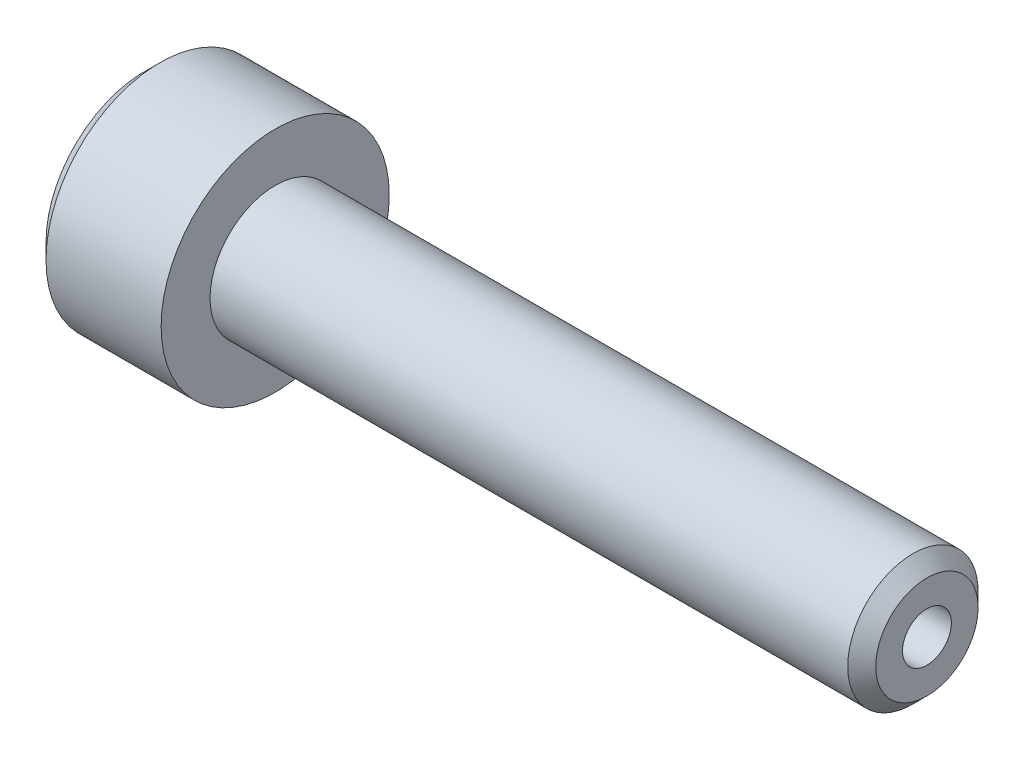
from build123d import *

# Parameters (mm, degrees)
CUT_EXTRUDE1_DEPTH = 2


with BuildPart() as part:
    # Sketch1 → Revolve1 (revolve)
    with BuildSketch(Plane.XY, mode=Mode.PRIVATE) as revolve1_sk:
        Polygon((-4, 0), (-4, 3.033333333), (-3.533333333, 3.5), (0, 3.5), (0, 2), (19.5699655, 2), (20, 1.5699655), (20, 0), align=None)
    revolve(revolve1_sk.sketch.rotate(Axis((20, 0, 0), (-1, 0, 0)), 270), axis=Axis((20, 0, 0), (-1, 0, 0)))

    # Sketch2 → Cut-Revolve1 (revolve, cut)
    with BuildSketch(Plane.XY, mode=Mode.PRIVATE) as cut_revolve1_sk:
        Polygon((-4, 0), (-4, 1.5), (-2, 1.5), (-1.727022324, 0.75), (20, 0.75), (20, 0), align=None)
    revolve(cut_revolve1_sk.sketch.rotate(Axis((20, 0, 0), (-1, 0, 0)), 270), axis=Axis((20, 0, 0), (-1, 0, 0)), mode=Mode.SUBTRACT)

    # Sketch3 → Cut-Extrude1 (cut)
    with BuildSketch(Plane(origin=(-4, 0, 0), x_dir=(0, 0, -1), z_dir=(1, 0, 0))):
        Polygon((-1.5, 0.866025404), (-1.5, -0.866025404), (0, -1.732050808), (1.5, -0.866025404), (1.5, 0.866025404), (0, 1.732050808), align=None)
    extrude(amount=CUT_EXTRUDE1_DEPTH, mode=Mode.SUBTRACT)


solid = part.part
